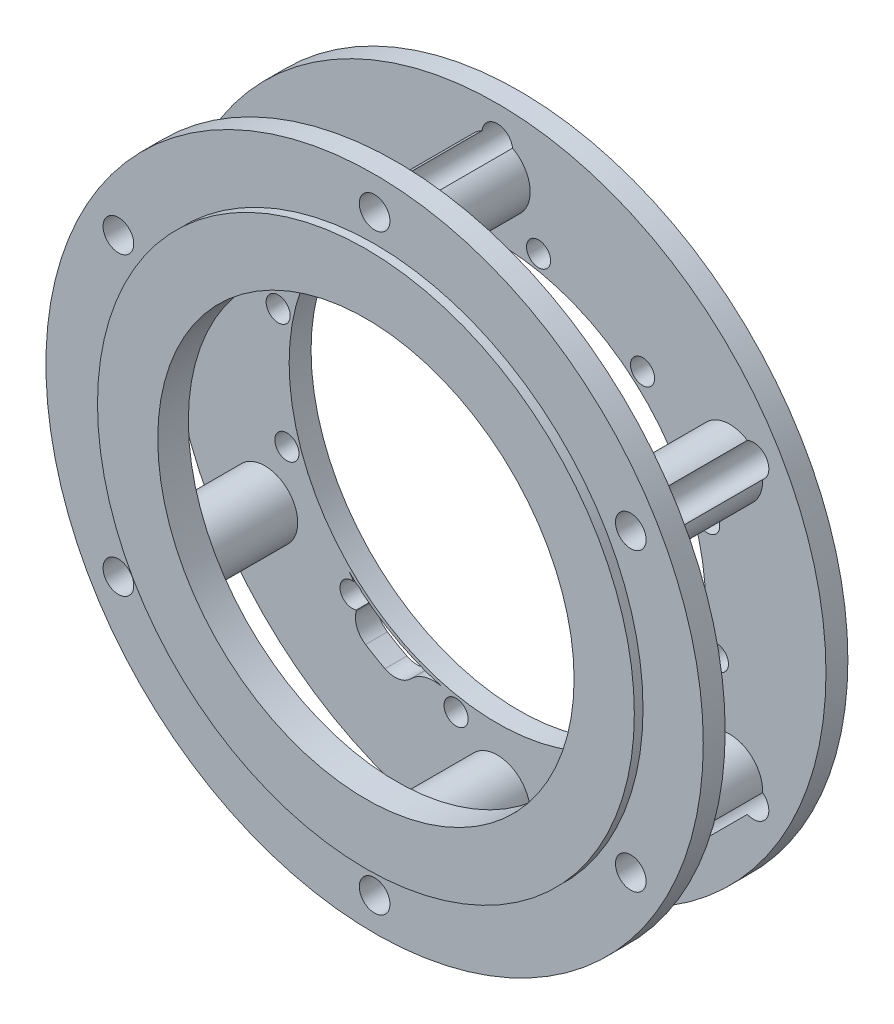
SolidWorks part; units mm, degrees
ref_plane "Front Plane" through (0, 0, 0) normal (0, 0, 1) x (1, 0, 0)
ref_plane "Top Plane" through (0, 0, 0) normal (0, 1, 0) x (1, 0, 0)
ref_plane "Right Plane" through (0, 0, 0) normal (1, 0, 0) x (0, 0, -1)
other "Configuration Table"
sketch "Sketch1" plane through (0, 0, 0) normal (0, 0, 1) x (1, 0, 0)
  circle A0 centre (0, 0) radius 150
  dimension "D1" = 300
extrude "Boss-Extrude1" add sketch "Sketch1" along normal blind 10
sketch "Sketch2" plane through (0, 0, 10) normal (0, 0, 1) x (1, 0, 0)
  circle A0 centre (0, 0) radius 122.5 construction
  circle A1 centre (0, 122.5) radius 15
  circle A2 centre (106.0881, 61.25) radius 15
  circle A3 centre (106.0881, -61.25) radius 15
  circle A4 centre (0, -122.5) radius 15
  circle A5 centre (-106.0881, -61.25) radius 15
  circle A6 centre (-106.0881, 61.25) radius 15
  point P18 (0, 0)
  dimension "D1" = 245
  dimension "D2" = 30
  dimension "D3" = 6
extrude "Boss-Extrude2" add sketch "Sketch2" along normal blind 46
sketch "Sketch3" plane through (0, 0, 56) normal (0, 0, 1) x (1, 0, 0)
  circle A0 centre (0, 0) radius 150
  dimension "D1" = 300
extrude "Boss-Extrude3" add sketch "Sketch3" along normal blind 10
sketch "Sketch4" plane through (0, 0, 66) normal (0, 0, 1) x (1, 0, 0)
  circle A0 centre (0, 0) radius 122.5
  dimension "D1" = 245
extrude "Boss-Extrude4" add sketch "Sketch4" along normal blind 3.96
sketch "Sketch5" plane through (0, 0, 0) normal (0, 0, -1) x (-1, 0, 0)
  circle A0 centre (0, 0) radius 135 construction
  circle A1 centre (0, 135) radius 7
  circle A2 centre (116.9134, 67.5) radius 7
  circle A3 centre (116.9134, -67.5) radius 7
  circle A4 centre (0, -135) radius 7
  circle A5 centre (-116.9134, -67.5) radius 7
  circle A6 centre (-116.9134, 67.5) radius 7
  point P18 (0, 0)
  dimension "D1" = 270
  dimension "D2" = 14
  dimension "D3" = 6
extrude "Cut-Extrude2" cut sketch "Sketch5" against normal up to surface (69.96 mm away) up to face at (122.5, 0, 69.96)
sketch "Sketch6" plane through (0, 0, 0) normal (0, 0, -1) x (-1, 0, 0)
  circle A0 centre (0, 0) radius 95
  dimension "D1" = 190
extrude "Cut-Extrude3" cut sketch "Sketch6" against normal up to surface (69.96 mm away) up to face at (122.5, 0, 69.96)
sketch "Sketch7" plane through (0, 0, 0) normal (0, 0, -1) x (-1, 0, 0)
  line L0 (0, 174.7093) -> (0, 0) construction
  line L1 (0, 0) -> (-41.1656, 153.6321) construction
  arc A0 (-51.2508, 99.0232) -> (-5.1271, 111.3821) centre (0, 0) ccw
  arc A1 (-39.5359, 97.1656) -> (-14.3437, 103.9159) centre (-28.8583, 107.7007) ccw
  arc A2 (-39.5359, 97.1656) -> (-51.2508, 99.0232) centre (-46.6544, 90.1422) ccw
  arc A3 (-14.3437, 103.9159) -> (-5.1271, 111.3821) centre (-4.6673, 101.3926) cw
  arc A4 (14.3437, 103.9159) -> (39.5359, 97.1656) centre (28.8583, 107.7007) ccw
  arc A5 (39.5359, 97.1656) -> (51.2508, 99.0232) centre (46.6544, 90.1422) cw
  arc A6 (14.3437, 103.9159) -> (5.1271, 111.3821) centre (4.6673, 101.3926) ccw
  arc A7 (64.3799, 82.8219) -> (82.8219, 64.3799) centre (78.8424, 78.8424) ccw
  arc A8 (82.8219, 64.3799) -> (93.8962, 60.1312) centre (85.475, 54.7383) cw
  arc A9 (64.3799, 82.8219) -> (60.1312, 93.8962) centre (54.7383, 85.475) ccw
  arc A10 (97.1656, 39.5359) -> (103.9159, 14.3437) centre (107.7007, 28.8583) ccw
  arc A11 (103.9159, 14.3437) -> (111.3821, 5.1271) centre (101.3926, 4.6673) cw
  arc A12 (97.1656, 39.5359) -> (99.0232, 51.2508) centre (90.1422, 46.6544) ccw
  arc A13 (103.9159, -14.3437) -> (97.1656, -39.5359) centre (107.7007, -28.8583) ccw
  arc A14 (97.1656, -39.5359) -> (99.0232, -51.2508) centre (90.1422, -46.6544) cw
  arc A15 (103.9159, -14.3437) -> (111.3821, -5.1271) centre (101.3926, -4.6673) ccw
  arc A16 (82.8219, -64.3799) -> (64.3799, -82.8219) centre (78.8424, -78.8424) ccw
  arc A17 (64.3799, -82.8219) -> (60.1312, -93.8962) centre (54.7383, -85.475) cw
  arc A18 (82.8219, -64.3799) -> (93.8962, -60.1312) centre (85.475, -54.7383) ccw
  arc A19 (39.5359, -97.1656) -> (14.3437, -103.9159) centre (28.8583, -107.7007) ccw
  arc A20 (14.3437, -103.9159) -> (5.1271, -111.3821) centre (4.6673, -101.3926) cw
  arc A21 (39.5359, -97.1656) -> (51.2508, -99.0232) centre (46.6544, -90.1422) ccw
  arc A22 (-14.3437, -103.9159) -> (-39.5359, -97.1656) centre (-28.8583, -107.7007) ccw
  arc A23 (-39.5359, -97.1656) -> (-51.2508, -99.0232) centre (-46.6544, -90.1422) cw
  arc A24 (-14.3437, -103.9159) -> (-5.1271, -111.3821) centre (-4.6673, -101.3926) ccw
  arc A25 (-64.3799, -82.8219) -> (-82.8219, -64.3799) centre (-78.8424, -78.8424) ccw
  arc A26 (-82.8219, -64.3799) -> (-93.8962, -60.1312) centre (-85.475, -54.7383) cw
  arc A27 (-64.3799, -82.8219) -> (-60.1312, -93.8962) centre (-54.7383, -85.475) ccw
  arc A28 (-97.1656, -39.5359) -> (-103.9159, -14.3437) centre (-107.7007, -28.8583) ccw
  arc A29 (-103.9159, -14.3437) -> (-111.3821, -5.1271) centre (-101.3926, -4.6673) cw
  arc A30 (-97.1656, -39.5359) -> (-99.0232, -51.2508) centre (-90.1422, -46.6544) ccw
  arc A31 (-103.9159, 14.3437) -> (-97.1656, 39.5359) centre (-107.7007, 28.8583) ccw
  arc A32 (-97.1656, 39.5359) -> (-99.0232, 51.2508) centre (-90.1422, 46.6544) cw
  arc A33 (-103.9159, 14.3437) -> (-111.3821, 5.1271) centre (-101.3926, 4.6673) ccw
  arc A34 (-82.8219, 64.3799) -> (-64.3799, 82.8219) centre (-78.8424, 78.8424) ccw
  arc A35 (-64.3799, 82.8219) -> (-60.1312, 93.8962) centre (-54.7383, 85.475) cw
  arc A36 (-82.8219, 64.3799) -> (-93.8962, 60.1312) centre (-85.475, 54.7383) ccw
  circle A37 centre (0, 0) radius 96.5
  point P91 (0, 0)
  dimension "D1" = 223
  dimension "D3" = 30
  dimension "D4" = 10
  dimension "D2" = 15
  dimension "D5" = 12
extrude "Cut-Extrude9" cut sketch "Sketch7" against normal up to surface (10 mm away) contours A37 A19 A21 A0 A17 A16 up to face at (95, 0, 10)
sketch "Sketch8" plane through (0, 0, 0) normal (0, 0, -1) x (-1, 0, 0)
  circle A0 centre (0, 0) radius 101.75 construction
  circle A1 centre (18.8179, -99.9947) radius 5.5
  circle A2 centre (-33.7006, -96.0069) radius 5.5
  circle A3 centre (-77.189, -66.2942) radius 5.5
  circle A4 centre (-99.9947, -18.8179) radius 5.5
  circle A5 centre (-96.0069, 33.7006) radius 5.5
  circle A6 centre (-66.2942, 77.189) radius 5.5
  circle A7 centre (-18.8179, 99.9947) radius 5.5
  circle A8 centre (33.7006, 96.0069) radius 5.5
  circle A9 centre (77.189, 66.2942) radius 5.5
  circle A10 centre (99.9947, 18.8179) radius 5.5
  circle A11 centre (96.0069, -33.7006) radius 5.5
  circle A12 centre (66.2942, -77.189) radius 5.5
  point P30 (0, 0)
  dimension "D1" = 203.5
  dimension "D2" = 11
  dimension "D3" = 12
extrude "Cut-Extrude10" cut sketch "Sketch8" against normal up to surface (10 mm away) up to face at (95, 0, 10)
